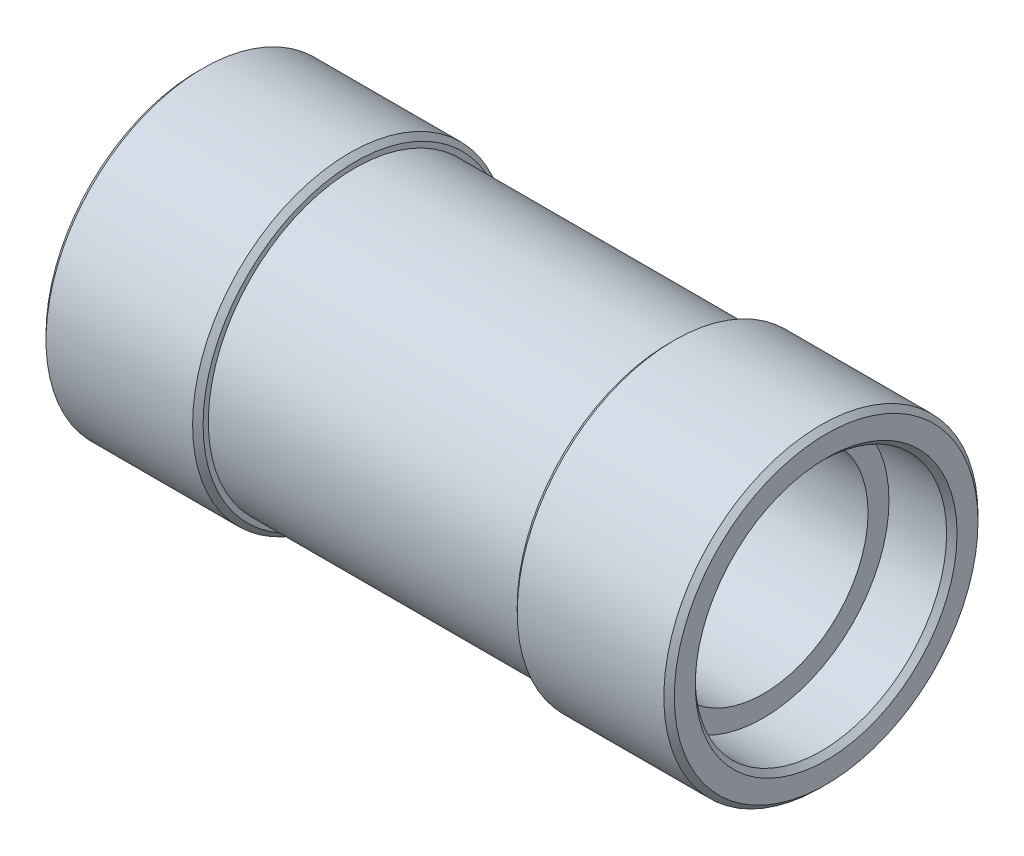
from build123d import *

# Parameters (mm, degrees)
CHAMFER1_SIZE = 0.5


with BuildPart() as part:
    # Sketch1 → Revolve1 (revolve)
    with BuildSketch(Plane.XY, mode=Mode.PRIVATE) as revolve1_sk:
        Polygon((-24, 12), (-24, 10), (24, 10), (24, 12), (30, 12), (30, 15), (15, 15), (15, 14), (-15, 14), (-15, 15), (-30, 15), (-30, 12), align=None)
    revolve(revolve1_sk.sketch.rotate(Axis((48.533661203, 0, 0), (-1, 0, 0)), 90), axis=Axis((48.533661203, 0, 0), (-1, 0, 0)))

    # Chamfer1
    chamfer1_edges = [part.edges().sort_by_distance(p)[0] for p in [
        (30, 0, 12),
        (-30, 0, 12),
        (-30, 0, 15),
        (-15, 0, 15),
        (15, 0, 15),
        (30, 0, 15),
    ]]
    chamfer(chamfer1_edges, length=CHAMFER1_SIZE)


solid = part.part
